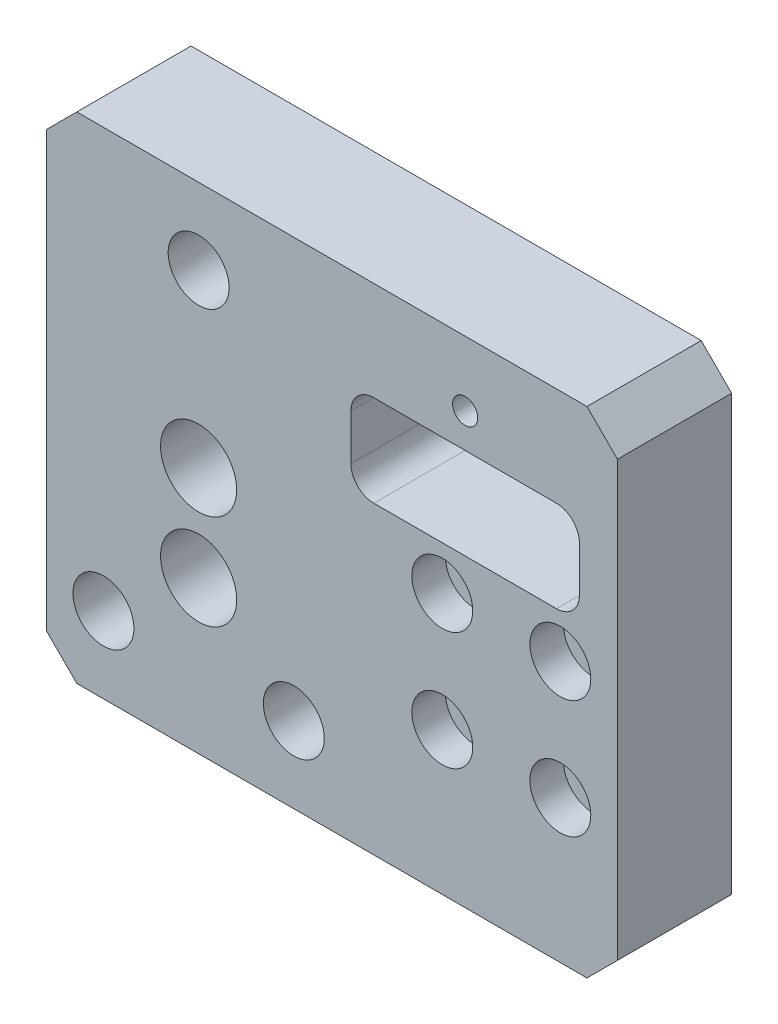
SolidWorks part; units mm, degrees
material "SUS304"
ref_plane "前视基准面" through (0, 0, 0) normal (0, 0, 1) x (1, 0, 0)
ref_plane "上视基准面" through (0, 0, 0) normal (0, 1, 0) x (1, 0, 0)
ref_plane "右视基准面" through (0, 0, 0) normal (1, 0, 0) x (0, 0, -1)
sketch "草图1" plane through (0, 0, 0) normal (0, 0, 1) x (1, 0, 0)
  line L1 (-37.5, -32.5) -> (37.5, -32.5)
  line L2 (-37.5, -32.5) -> (-37.5, 32.5)
  line L3 (-37.5, 32.5) -> (37.5, 32.5)
  line L4 (37.5, -32.5) -> (37.5, 32.5)
  line L5 (-37.5, -32.5) -> (37.5, 32.5) construction
  line L6 (-37.5, 32.5) -> (37.5, -32.5) construction
  point P0 (0, 0)
  dimension "D1" = 75
  dimension "D2" = 65
extrude "凸台-拉伸1" add sketch "草图1" along normal mid plane 15
hole_wizard "M4 六角凹头螺钉的柱形沉头孔1" positions "草图3" profile "草图2" counterbore size "M4" standard "ISO" end condition through all
sketch "草图3" plane through (0, 0, 7.5) normal (0, 0, 1) x (1, 0, 0)
  line L2 (-37.5, -32.5) -> (37.5, -32.5) construction
  line L3 (-37.5, 32.5) -> (-37.5, -32.5) construction
  point P0 (14.5, 1.75)
  point P2 (14.5, -13.75)
  point P4 (30, 1.75)
  point P6 (30, -13.75)
  dimension "D1" = 15.5
  dimension "D2" = 52
  dimension "D4" = 18.75
  dimension "D5" = 34.25
sketch "草图2" plane through (14.5, 1.75, 7.5) normal (1, 0, 0) x (0, -1, 0)
  line L0 (0, 0) -> (0, 15)
  line L1 (0, 15) -> (2.25, 15)
  line L3 (2.25, 15) -> (2.25, 4.4)
  line L4 (2.25, 4.4) -> (4, 4.4)
  line L5 (4, 4.4) -> (4, 0)
  line L7 (4, 0) -> (0, 0)
  line L11 (0, -6.35) -> (0, 107.95) construction
  dimension "通孔孔直径" = 4.5
  dimension "通孔孔深度" = 15
  dimension "柱形沉头孔直径" = 8
  dimension "柱形沉头孔深度" = 4.4
hole_wizard "Ø8.0 (8) 直径孔1" positions "草图5" profile "草图4" hole size "Ø8.0" standard "ISO" end condition through all
sketch "草图5" plane through (0, 0, 7.5) normal (0, 0, 1) x (1, 0, 0)
  line L1 (-37.5, -32.5) -> (37.5, -32.5) construction
  line L2 (-17.5, 22.5) -> (-17.5, -22.5) construction
  line L3 (-37.5, 32.5) -> (-37.5, -32.5) construction
  point P0 (-17.5, 22.5)
  point P2 (-30, -22.5)
  point P4 (-5, -22.5)
  dimension "D1" = 25
  dimension "D2" = 20
  dimension "D3" = 12.5
  dimension "D4" = 10
  dimension "D5" = 55
sketch "草图4" plane through (-17.5, 22.5, 7.5) normal (1, 0, 0) x (0, -1, 0)
  line L0 (0, 0) -> (0, 15)
  line L1 (0, 15) -> (4, 15)
  line L2 (4, 15) -> (4, 0)
  line L5 (4, 0) -> (0, 0)
  line L11 (0, -6.35) -> (0, 107.95) construction
  dimension "通孔孔直径" = 8
  dimension "通孔孔深度" = 15
hole_wizard "孔1" positions "草图7" profile "草图6" legacy end condition through all
sketch "草图7" plane through (0, 0, 7.5) normal (0, 0, 1) x (1, 0, 0)
  line L2 (-17.5, 22.5) -> (-17.5, 0) construction
  circle A0 centre (-5, -22.5) radius 4 construction
  point P0 (-17.5, 0)
  point P2 (-17.5, -12.5)
  dimension "D1" = 10
  dimension "D2" = 12.5
sketch "草图6" plane through (-17.5, 0, 7.5) normal (1, 0, 0) x (0, -1, 0)
  line L0 (0, 0) -> (0, 15)
  line L1 (0, 15) -> (2.25, 15)
  line L2 (2.25, 15) -> (2.25, 7.5)
  line L3 (2.25, 7.5) -> (5, 7.5)
  line L4 (5, 7.5) -> (5, 0)
  line L5 (5, 0) -> (0, 0)
  line L6 (0, 110) -> (0, -10) construction
  dimension "直径" = 4.5
  dimension "深度" = 15
  dimension "柱坑直径" = 10
  dimension "柱坑深度" = 7.5
sketch "草图8" plane through (0, 0, -7.5) normal (0, 0, -1) x (-1, 0, 0)
  circle A0 centre (17.5, 0) radius 4
  circle A1 centre (17.5, -12.5) radius 4
  dimension "D1" = 8
extrude "切除-拉伸1" cut sketch "草图8" against normal blind 4.5
chamfer "倒角1" distance 4 angle 45 4 edges at (-37.5, -32.5, 0) (37.5, -32.5, 0) (37.5, 32.5, 0) (-37.5, 32.5, 0)
sketch "草图9" plane through (0, 0, -7.5) normal (0, 0, -1) x (-1, 0, 0)
  line L0 (-9.5, 13.5) -> (-29.5, 13.5) construction
  line L1 (-2.5, 7.5) -> (-32.5, 7.5)
  line L2 (-2.5, 19.5) -> (-32.5, 19.5)
  line L3 (-37.5, -28.5) -> (-37.5, 28.5) construction
  line L4 (-33.5, 32.5) -> (33.5, 32.5) construction
  line L5 (-32.5, 19.5) -> (-32.5, 7.5)
  line L6 (-2.5, 19.5) -> (-2.5, 7.5)
  point P2 (-19.5, 15.5)
  dimension "D3" = 5
  dimension "D1" = 30
  dimension "D2" = 12
  dimension "D4" = 19
extrude "切除-拉伸2" cut sketch "草图9" against normal through all
hole_wizard "M4 螺纹孔1" positions "草图10" profile "草图12" tap size "M4" standard "GB" end condition through all
sketch "草图10" plane through (0, 0, -7.5) normal (0, 0, -1) x (-1, 0, 0)
  line L1 (-2.5, 19.5) -> (-32.5, 19.5) construction
  line L2 (-17.5, 19.5) -> (-17.5, 24) construction
  point P0 (-17.5, 24)
  dimension "D2" = 4.5
sketch "草图12" plane through (17.5, 24, -7.5) normal (1, 0, 0) x (0, 1, 0)
  line L0 (0, 0) -> (0, 15)
  line L1 (0, 15) -> (1.65, 15)
  line L2 (1.65, 15) -> (1.65, 0)
  line L5 (1.65, 0) -> (0, 0)
  line L11 (0, -6.35) -> (0, 107.95) construction
  dimension "通孔螺纹孔钻头直径" = 3.3
  dimension "通孔螺纹孔钻头深度" = 15
cosmetic thread "孔螺蚊线1" parameters "D2"=4
fillet "圆角1" radius 3 4 edges at (2.5, 7.5, 0) (32.5, 7.5, 0) (2.5, 19.5, 0) (32.5, 19.5, 0)
